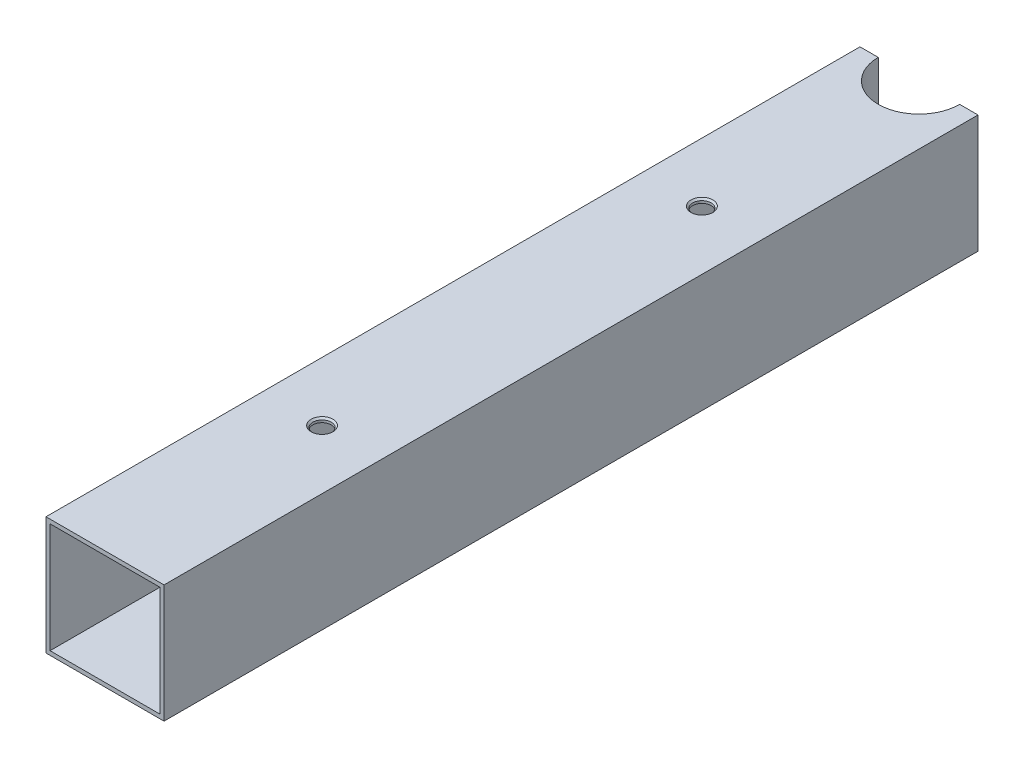
from build123d import *

# Parameters (mm, degrees)
SKETCH1_W                   = 43.5
SKETCH1_H                   = 43.5
SKETCH1_W_2                 = 40.5
SKETCH1_H_2                 = 40.5
BOSS_EXTRUDE1_DEPTH         = 300
SKETCH2_W                   = 43.5
SKETCH2_H                   = 43.5
BOSS_EXTRUDE2_DEPTH         = 30
M8_TAPPED_HOLE1_D           = 6.8
M8_TAPPED_HOLE1_CSINK_D     = 8.05
M8_TAPPED_HOLE1_CSINK_ANGLE = 90
CUT_EXTRUDE1_DEPTH          = 307.033086447
SKETCH6_R                   = 5
CUT_EXTRUDE2_DEPTH          = 306.823478497


with BuildPart() as part:
    # Sketch1 → Boss-Extrude1 (new body)
    with BuildSketch(Plane.XY):
        with Locations((-20.25, 20.25)):
            Rectangle(SKETCH1_W, SKETCH1_H)
        with Locations((-20.25, 20.25)):
            Rectangle(SKETCH1_W_2, SKETCH1_H_2, mode=Mode.SUBTRACT)
    extrude(amount=BOSS_EXTRUDE1_DEPTH)

    # Sketch2 → Boss-Extrude2 (add)
    with BuildSketch(Plane(origin=(0, 0, 0), x_dir=(-1, 0, 0), z_dir=(0, 0, -1))):
        with Locations((20.25, 20.25)):
            Rectangle(SKETCH2_W, SKETCH2_H)
    extrude(amount=-BOSS_EXTRUDE2_DEPTH)

    # M8 Tapped Hole1 (through all)
    with Locations(Plane(origin=(0, 42, 0), x_dir=(1, 0, 0), z_dir=(0, 1, 0))):
        with Locations((-20.25, -220), (-20.25, -80)):
            CounterSinkHole(M8_TAPPED_HOLE1_D / 2, M8_TAPPED_HOLE1_CSINK_D / 2, counter_sink_angle=M8_TAPPED_HOLE1_CSINK_ANGLE)

    # Sketch5 → Cut-Extrude1 (cut, through all)
    with BuildSketch(Plane(origin=(0, 42, 0), x_dir=(1, 0, 0), z_dir=(0, 1, 0))):
        with BuildLine():
            Line((-35.25, 0), (-5.25, 0))
            ThreePointArc((-5.25, 0), (-20.25, -15), (-35.25, 0))
        make_face()
    extrude(amount=-CUT_EXTRUDE1_DEPTH, mode=Mode.SUBTRACT)

    # Sketch6 → Cut-Extrude2 (cut, through all)
    with BuildSketch(Plane(origin=(0, 0, 0), x_dir=(-1, 0, 0), z_dir=(0, 0, -1))):
        with Locations((20.25, 20.25)):
            Circle(SKETCH6_R)
    extrude(amount=-CUT_EXTRUDE2_DEPTH, mode=Mode.SUBTRACT)


solid = part.part
